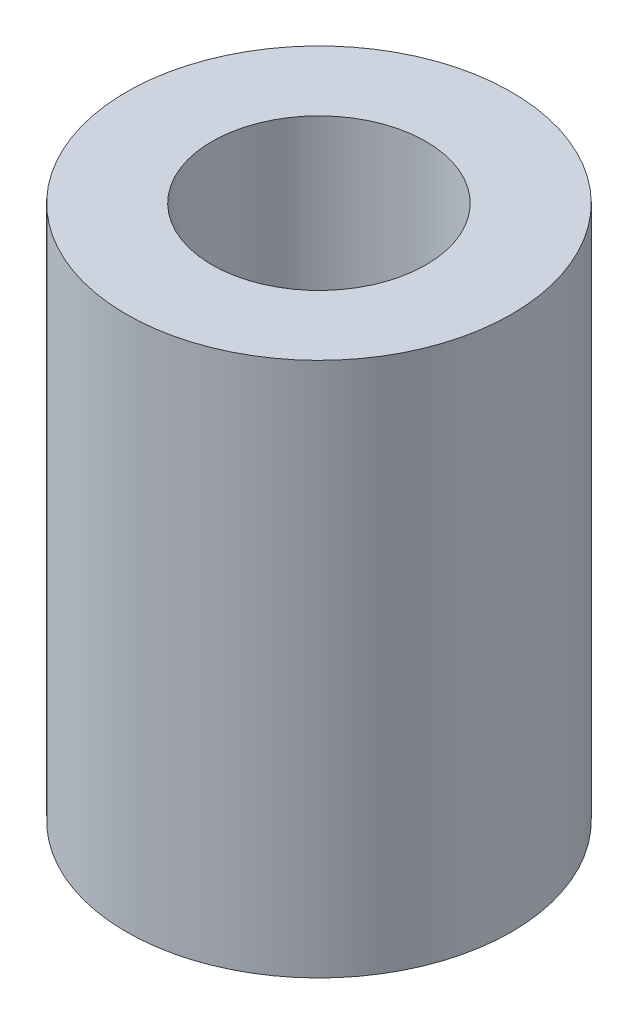
from build123d import *

# Parameters (mm, degrees)
SKETCH1_W = 4
SKETCH1_H = 25


with BuildPart() as part:
    # Sketch1 → Revolve1 (revolve)
    with BuildSketch(Plane.XY):
        with Locations((7, 12.5)):
            Rectangle(SKETCH1_W, SKETCH1_H)
    revolve(axis=Axis((0, -309.731791339, 0), (0, 1, 0)))


solid = part.part
